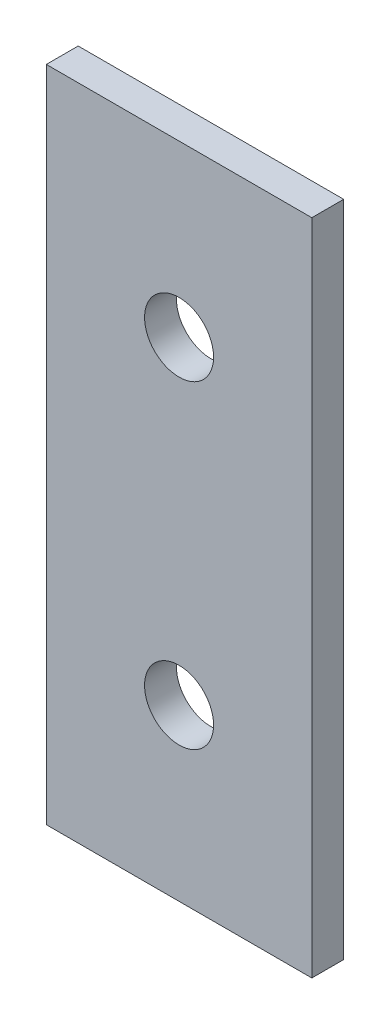
SolidWorks part; units mm, degrees
material "普通碳钢"
ref_plane "Front Plane" through (0, 0, 0) normal (0, 0, 1) x (1, 0, 0)
ref_plane "Top Plane" through (0, 0, 0) normal (0, 1, 0) x (1, 0, 0)
ref_plane "Right Plane" through (0, 0, 0) normal (1, 0, 0) x (0, 0, -1)
sketch "Sketch1" plane through (0, 0, 0) normal (0, 0, 1) x (1, 0, 0)
  line L2 (25, -62) -> (25, 62)
  line L3 (25, 62) -> (-25, 62)
  line L4 (-25, 62) -> (-25, -62)
  line L5 (-25, -62) -> (25, -62)
  dimension "D1" = 124
  dimension "D2" = 50
extrude "Extrude1" add sketch "Sketch1" along normal mid plane 6
sketch "Sketch2" plane through (0, 0, 3) normal (0, 0, 1) x (1, 0, 0)
  line L0 (0, 30) -> (0, -30) construction
  circle A0 centre (0, 30) radius 6.5
  circle A1 centre (0, -30) radius 6.5
  dimension "D1" = 13
  dimension "D2" = 13
  dimension "D3" = 30
  dimension "D4" = 30
extrude "Cut-Extrude1" cut sketch "Sketch2" against normal blind 22
